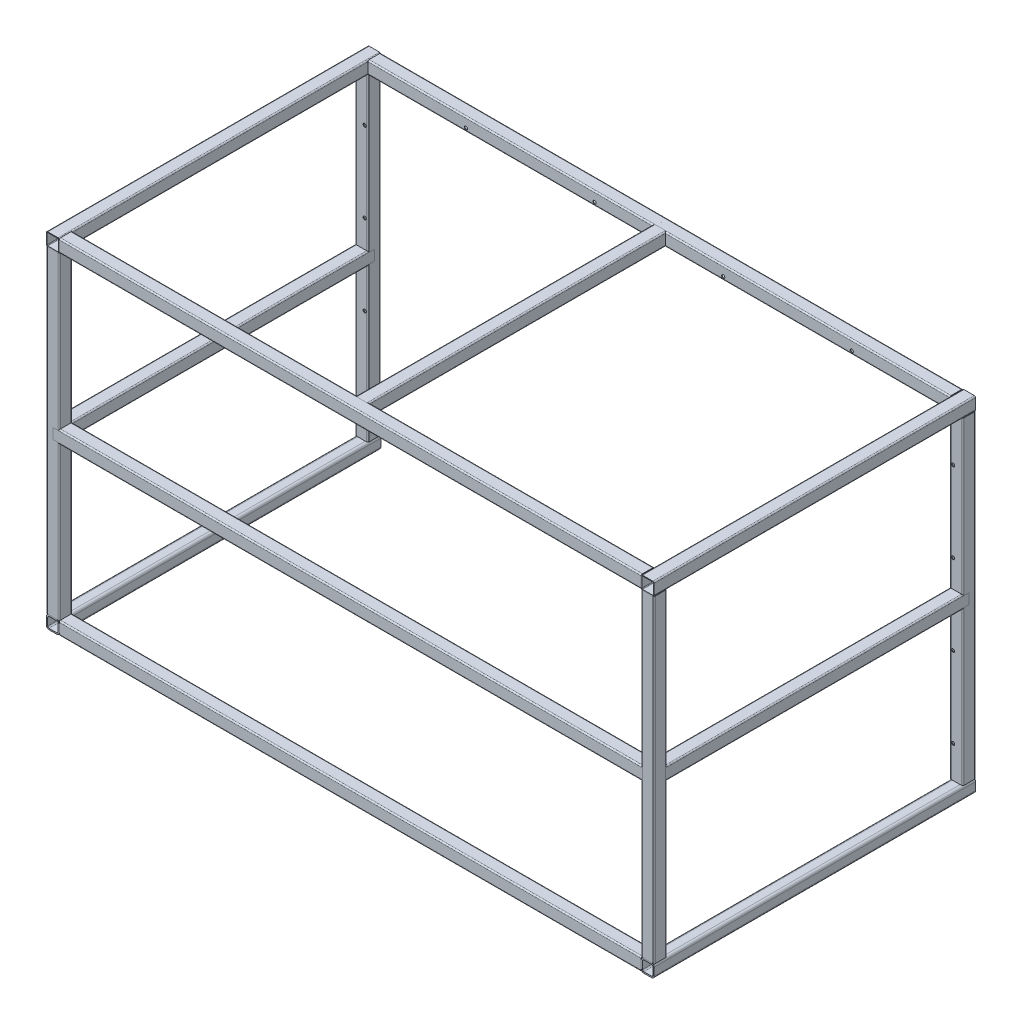
SolidWorks part; units mm, degrees
ref_plane "前视基准面" through (0, 0, 0) normal (0, 0, 1) x (1, 0, 0)
ref_plane "上视基准面" through (0, 0, 0) normal (0, 1, 0) x (1, 0, 0)
ref_plane "右视基准面" through (0, 0, 0) normal (1, 0, 0) x (0, 0, -1)
sketch "草图1" plane through (0, 0, 0) normal (0, 0, 1) x (1, 0, 0)
  line L1 (-925, -515) -> (925, -515)
  line L2 (-925, -515) -> (-925, 515)
  line L3 (-925, 515) -> (925, 515)
  line L4 (925, -515) -> (925, 515)
  line L5 (-925, -515) -> (925, 515) construction
  line L6 (-925, 515) -> (925, -515) construction
  point P0 (0, 0)
  dimension "D1" = 1030
  dimension "D2" = 1850
ref_plane "基准面1" through (0, 0, -960) normal (0, 0, 1) x (1, 0, 0)
sketch "草图2" plane through (0, 0, -960) normal (0, 0, 1) x (1, 0, 0)
  line L0 (-925, -515) -> (925, -515) construction
  line L1 (925, -515) -> (925, 515) construction
  line L2 (-925, 515) -> (925, 515) construction
  line L3 (-925, -515) -> (-925, 515) construction
  line L4 (-925, -515) -> (925, -515)
  line L5 (925, -515) -> (925, 515)
  line L6 (-925, 515) -> (925, 515)
  line L7 (-925, -515) -> (-925, 515)
sketch3d "3D草图1"
  line L0 (-925, -515, 0) -> (-925, -515, -960)
  line L1 (925, -515, 0) -> (925, -515, -960)
  line L2 (-925, 515, 0) -> (-925, 515, -960)
  line L3 (925, 515, 0) -> (925, 515, -960)
  line L4 (925, -515, -660) -> (925, 515, -660)
  dimension "D1" = 300
other "Square tube - configured 40 X 40 X 4(1)"
ref_plane "基准面2" through (-925, 515, 0) normal (1, 0, 0) x (0, 1, 0)
sketch "Sketch1" plane through (-925, 515, 0) normal (1, 0, 0) x (0, 1, 0)
  line L0 (-16, -18) -> (16, -18)
  line L1 (-18, -16) -> (-18, 16)
  line L2 (16, 18) -> (-16, 18)
  line L3 (18, 16) -> (18, -16)
  line L4 (-16, -20) -> (16, -20)
  line L5 (-20, -16) -> (-20, 16)
  line L6 (16, 20) -> (-16, 20)
  line L7 (20, 16) -> (20, -16)
  arc A0 (20, 16) -> (16, 20) centre (16, 16) ccw
  arc A1 (16, -20) -> (20, -16) centre (16, -16) ccw
  arc A2 (-20, -16) -> (-16, -20) centre (-16, -16) ccw
  arc A3 (-16, 20) -> (-20, 16) centre (-16, 16) ccw
  arc A4 (-16, 18) -> (-18, 16) centre (-16, 16) ccw
  arc A5 (18, 16) -> (16, 18) centre (16, 16) ccw
  arc A6 (16, -18) -> (18, -16) centre (16, -16) ccw
  arc A7 (-18, -16) -> (-16, -18) centre (-16, -16) ccw
  point P0 (-20, 0)
  point P1 (20, 0)
  point P2 (0, 20)
  point P3 (0, -20)
  point P4 (0, 0)
  point P5 (-20, -20)
  point P6 (20, -20)
  point P7 (20, 20)
  point P8 (-20, 20)
  point P33 (0, 0)
  dimension "D1" = 4
  dimension "Thickness" = 2
  dimension "V_leg" = 40
other "Square tube - configured 40 X 40 X 4(2)"
ref_plane "基准面3" through (925, -515, -960) normal (0, 1, 0) x (-1, 0, 0)
sketch "Sketch11" plane through (925, -515, -960) normal (0, 1, 0) x (-1, 0, 0)
  line L0 (-16, -18) -> (16, -18)
  line L1 (-18, -16) -> (-18, 16)
  line L2 (16, 18) -> (-16, 18)
  line L3 (18, 16) -> (18, -16)
  line L4 (-16, -20) -> (16, -20)
  line L5 (-20, -16) -> (-20, 16)
  line L6 (16, 20) -> (-16, 20)
  line L7 (20, 16) -> (20, -16)
  arc A0 (20, 16) -> (16, 20) centre (16, 16) ccw
  arc A1 (16, -20) -> (20, -16) centre (16, -16) ccw
  arc A2 (-20, -16) -> (-16, -20) centre (-16, -16) ccw
  arc A3 (-16, 20) -> (-20, 16) centre (-16, 16) ccw
  arc A4 (-16, 18) -> (-18, 16) centre (-16, 16) ccw
  arc A5 (18, 16) -> (16, 18) centre (16, 16) ccw
  arc A6 (16, -18) -> (18, -16) centre (16, -16) ccw
  arc A7 (-18, -16) -> (-16, -18) centre (-16, -16) ccw
  point P0 (-20, 0)
  point P1 (20, 0)
  point P2 (0, 20)
  point P3 (0, -20)
  point P4 (0, 0)
  point P5 (-20, -20)
  point P6 (20, -20)
  point P7 (20, 20)
  point P8 (-20, 20)
  point P33 (0, 0)
  dimension "D1" = 4
  dimension "Thickness" = 2
  dimension "V_leg" = 40
other "Square tube - configured 40 X 40 X 4(4)"
ref_plane "基准面4" through (-925, 515, 0) normal (0, 0, -1) x (1, 0, 0)
sketch "Sketch12" plane through (-925, 515, 0) normal (0, 0, -1) x (1, 0, 0)
  line L0 (-16, -18) -> (16, -18)
  line L1 (-18, -16) -> (-18, 16)
  line L2 (16, 18) -> (-16, 18)
  line L3 (18, 16) -> (18, -16)
  line L4 (-16, -20) -> (16, -20)
  line L5 (-20, -16) -> (-20, 16)
  line L6 (16, 20) -> (-16, 20)
  line L7 (20, 16) -> (20, -16)
  arc A0 (20, 16) -> (16, 20) centre (16, 16) ccw
  arc A1 (16, -20) -> (20, -16) centre (16, -16) ccw
  arc A2 (-20, -16) -> (-16, -20) centre (-16, -16) ccw
  arc A3 (-16, 20) -> (-20, 16) centre (-16, 16) ccw
  arc A4 (-16, 18) -> (-18, 16) centre (-16, 16) ccw
  arc A5 (18, 16) -> (16, 18) centre (16, 16) ccw
  arc A6 (16, -18) -> (18, -16) centre (16, -16) ccw
  arc A7 (-18, -16) -> (-16, -18) centre (-16, -16) ccw
  point P0 (-20, 0)
  point P1 (20, 0)
  point P2 (0, 20)
  point P3 (0, -20)
  point P4 (0, 0)
  point P5 (-20, -20)
  point P6 (20, -20)
  point P7 (20, 20)
  point P8 (-20, 20)
  point P33 (0, 0)
  dimension "D1" = 4
  dimension "Thickness" = 2
  dimension "V_leg" = 40
other "剪裁/延伸1"
other "剪裁/延伸5"
other "剪裁/延伸17"
other "剪裁/延伸18"
other "剪裁/延伸22"
other "剪裁/延伸23"
other "剪裁/延伸25"
sketch3d "3D草图2"
  line L0 (0, -515, -960) -> (0, -515, 0)
  line L1 (-925, -515, -960) -> (925, -515, -960) construction
  line L2 (-925, -515, 0) -> (925, -515, 0) construction
  line L3 (0, 515, -960) -> (0, 515, 0)
  line L4 (-925, 515, -960) -> (925, 515, -960) construction
  line L5 (-925, 515, 0) -> (925, 515, 0) construction
other "Square tube - configured 40 X 40 X 4(5)"
ref_plane "基准面6" through (0, 515, -960) normal (0, 0, 1) x (1, 0, 0)
sketch "Sketch14" plane through (0, 515, -960) normal (0, 0, 1) x (1, 0, 0)
  line L0 (-16, -18) -> (16, -18)
  line L1 (-18, -16) -> (-18, 16)
  line L2 (16, 18) -> (-16, 18)
  line L3 (18, 16) -> (18, -16)
  line L4 (-16, -20) -> (16, -20)
  line L5 (-20, -16) -> (-20, 16)
  line L6 (16, 20) -> (-16, 20)
  line L7 (20, 16) -> (20, -16)
  arc A0 (20, 16) -> (16, 20) centre (16, 16) ccw
  arc A1 (16, -20) -> (20, -16) centre (16, -16) ccw
  arc A2 (-20, -16) -> (-16, -20) centre (-16, -16) ccw
  arc A3 (-16, 20) -> (-20, 16) centre (-16, 16) ccw
  arc A4 (-16, 18) -> (-18, 16) centre (-16, 16) ccw
  arc A5 (18, 16) -> (16, 18) centre (16, 16) ccw
  arc A6 (16, -18) -> (18, -16) centre (16, -16) ccw
  arc A7 (-18, -16) -> (-16, -18) centre (-16, -16) ccw
  point P0 (-20, 0)
  point P1 (20, 0)
  point P2 (0, 20)
  point P3 (0, -20)
  point P4 (0, 0)
  point P5 (-20, -20)
  point P6 (20, -20)
  point P7 (20, 20)
  point P8 (-20, 20)
  point P33 (0, 0)
  dimension "D1" = 4
  dimension "Thickness" = 2
  dimension "V_leg" = 40
sketch3d "3D草图3"
  line L0 (925, 0, 0) -> (-925, 0, 0)
  line L1 (925, -515, 0) -> (925, 515, 0) construction
  line L2 (-925, -515, 0) -> (-925, 515, 0) construction
other "Square tube - configured 40 X 40 X 4(2)"
ref_plane "基准面7" through (925, 0, 0) normal (-1, 0, 0) x (0, 0, 1)
sketch "Sketch15" plane through (925, 0, 0) normal (-1, 0, 0) x (0, 0, 1)
  line L0 (-16, -18) -> (16, -18)
  line L1 (-18, -16) -> (-18, 16)
  line L2 (16, 18) -> (-16, 18)
  line L3 (18, 16) -> (18, -16)
  line L4 (-16, -20) -> (16, -20)
  line L5 (-20, -16) -> (-20, 16)
  line L6 (16, 20) -> (-16, 20)
  line L7 (20, 16) -> (20, -16)
  arc A0 (20, 16) -> (16, 20) centre (16, 16) ccw
  arc A1 (16, -20) -> (20, -16) centre (16, -16) ccw
  arc A2 (-20, -16) -> (-16, -20) centre (-16, -16) ccw
  arc A3 (-16, 20) -> (-20, 16) centre (-16, 16) ccw
  arc A4 (-16, 18) -> (-18, 16) centre (-16, 16) ccw
  arc A5 (18, 16) -> (16, 18) centre (16, 16) ccw
  arc A6 (16, -18) -> (18, -16) centre (16, -16) ccw
  arc A7 (-18, -16) -> (-16, -18) centre (-16, -16) ccw
  point P0 (-20, 0)
  point P1 (20, 0)
  point P2 (0, 20)
  point P3 (0, -20)
  point P4 (0, 0)
  point P5 (-20, -20)
  point P6 (20, -20)
  point P7 (20, 20)
  point P8 (-20, 20)
  point P33 (0, 0)
  dimension "D1" = 4
  dimension "Thickness" = 2
  dimension "V_leg" = 40
sketch3d "3D草图4"
  line L0 (-925, 0, 0) -> (-925, 0, -960)
  line L1 (-925, -515, 0) -> (-925, 515, 0) construction
  line L2 (-925, -515, -960) -> (-925, 515, -960) construction
  line L4 (-925, 515, 0) -> (-925, 515, -960) construction
  line L5 (925, 0, 0) -> (925, 0, -960)
  line L6 (925, -515, 0) -> (925, 515, 0) construction
  line L7 (925, -515, -960) -> (925, 515, -960) construction
  line L8 (925, 515, 0) -> (925, 515, -960) construction
  dimension "D1" = 515
  dimension "D2" = 515
other "Square tube - configured 40 X 40 X 4(5)"
ref_plane "基准面8" through (-925, 0, 0) normal (0, 0, -1) x (1, 0, 0)
sketch "Sketch16" plane through (-925, 0, 0) normal (0, 0, -1) x (1, 0, 0)
  line L0 (-16, -18) -> (16, -18)
  line L1 (-18, -16) -> (-18, 16)
  line L2 (16, 18) -> (-16, 18)
  line L3 (18, 16) -> (18, -16)
  line L4 (-16, -20) -> (16, -20)
  line L5 (-20, -16) -> (-20, 16)
  line L6 (16, 20) -> (-16, 20)
  line L7 (20, 16) -> (20, -16)
  arc A0 (20, 16) -> (16, 20) centre (16, 16) ccw
  arc A1 (16, -20) -> (20, -16) centre (16, -16) ccw
  arc A2 (-20, -16) -> (-16, -20) centre (-16, -16) ccw
  arc A3 (-16, 20) -> (-20, 16) centre (-16, 16) ccw
  arc A4 (-16, 18) -> (-18, 16) centre (-16, 16) ccw
  arc A5 (18, 16) -> (16, 18) centre (16, 16) ccw
  arc A6 (16, -18) -> (18, -16) centre (16, -16) ccw
  arc A7 (-18, -16) -> (-16, -18) centre (-16, -16) ccw
  point P0 (-20, 0)
  point P1 (20, 0)
  point P2 (0, 20)
  point P3 (0, -20)
  point P4 (0, 0)
  point P5 (-20, -20)
  point P6 (20, -20)
  point P7 (20, 20)
  point P8 (-20, 20)
  point P33 (0, 0)
  dimension "D1" = 4
  dimension "Thickness" = 2
  dimension "V_leg" = 40
sketch3d "3D草图5"
  line L0 (-925, -515, 0) -> (-925, -515, -670)
  line L1 (925, -515, 0) -> (925, -515, -670)
  line L2 (-925, -515, 0) -> (925, -515, 0) construction
  line L3 (-925, 515, 0) -> (925, -515, 0) construction
  dimension "D1" = 670
  dimension "D2" = 670
other "Square tube - configured 40 X 40 X 4(4)"
ref_plane "基准面9" through (-925, -515, 0) normal (0, 0, -1) x (1, 0, 0)
sketch "Sketch17" plane through (-925, -515, 0) normal (0, 0, -1) x (1, 0, 0)
  line L0 (-12, -16) -> (12, -16)
  line L1 (-16, -12) -> (-16, 12)
  line L2 (12, 16) -> (-12, 16)
  line L3 (16, 12) -> (16, -12)
  line L4 (-12, -20) -> (12, -20)
  line L5 (-20, -12) -> (-20, 12)
  line L6 (12, 20) -> (-12, 20)
  line L7 (20, 12) -> (20, -12)
  arc A0 (20, 12) -> (12, 20) centre (12, 12) ccw
  arc A1 (12, -20) -> (20, -12) centre (12, -12) ccw
  arc A2 (-20, -12) -> (-12, -20) centre (-12, -12) ccw
  arc A3 (-12, 20) -> (-20, 12) centre (-12, 12) ccw
  arc A4 (-12, 16) -> (-16, 12) centre (-12, 12) ccw
  arc A5 (16, 12) -> (12, 16) centre (12, 12) ccw
  arc A6 (12, -16) -> (16, -12) centre (12, -12) ccw
  arc A7 (-16, -12) -> (-12, -16) centre (-12, -12) ccw
  point P0 (-20, 0)
  point P1 (20, 0)
  point P2 (0, 20)
  point P3 (0, -20)
  point P4 (0, 0)
  point P5 (-20, -20)
  point P6 (20, -20)
  point P7 (20, 20)
  point P8 (-20, 20)
  point P33 (0, 0)
  dimension "D1" = 8
  dimension "Thickness" = 4
  dimension "V_leg" = 40
other "剪裁/延伸31"
other "剪裁/延伸32"
other "剪裁/延伸33"
other "剪裁/延伸34"
hole_wizard "Ø10.0 (10) 直径孔1" positions "草图3" profile "草图4" hole size "Ø10.0" standard "GB" end condition through all
sketch "草图3" plane through (0, 0, -940) normal (0, 0, 1) x (1, 0, 0)
  line L0 (945, 495) -> (945, -495) construction
  line L1 (941, -495) -> (909, -495) construction
  point P0 (915, -395)
  dimension "D1" = 30
  dimension "D2" = 100
sketch "草图4" plane through (915, -395, -940) normal (1, 0, 0) x (0, -1, 0)
  line L0 (0, 0) -> (0, 40)
  line L1 (0, 40) -> (5, 40)
  line L2 (5, 40) -> (5, 0)
  line L5 (5, 0) -> (0, 0)
  line L11 (0, -6.35) -> (0, 107.95) construction
  dimension "通孔孔直径" = 10
  dimension "通孔孔深度" = 40
pattern_linear "阵列(线性)1" count 4 spacing 250 along (0, 1, 0) of "Ø10.0 (10) 直径孔1"
pattern_linear "阵列(线性)2" count 2 spacing 1830 along (-1, 0, 0) of "Ø10.0 (10) 直径孔1", "阵列(线性)1"
hole_wizard "Ø10.0 (10) 直径孔2" positions "草图5" profile "草图6" hole size "Ø10.0" standard "GB" end condition through all
sketch "草图5" plane through (0, 0, -940) normal (0, 0, 1) x (1, 0, 0)
  line L0 (-905, 535) -> (905, 535) construction
  line L1 (905, 531) -> (905, 499) construction
  point P0 (600, 505)
  dimension "D1" = 30
  dimension "300" = 305
sketch "草图6" plane through (600, 505, -940) normal (1, 0, 0) x (0, -1, 0)
  line L0 (0, 0) -> (0, 40)
  line L1 (0, 40) -> (5, 40)
  line L2 (5, 40) -> (5, 0)
  line L5 (5, 0) -> (0, 0)
  line L11 (0, -6.35) -> (0, 107.95) construction
  dimension "通孔孔直径" = 10
  dimension "通孔孔深度" = 40
pattern_linear "阵列(线性)3" count 4 spacing 400 along (-1, 0, 0) of "Ø10.0 (10) 直径孔2"
